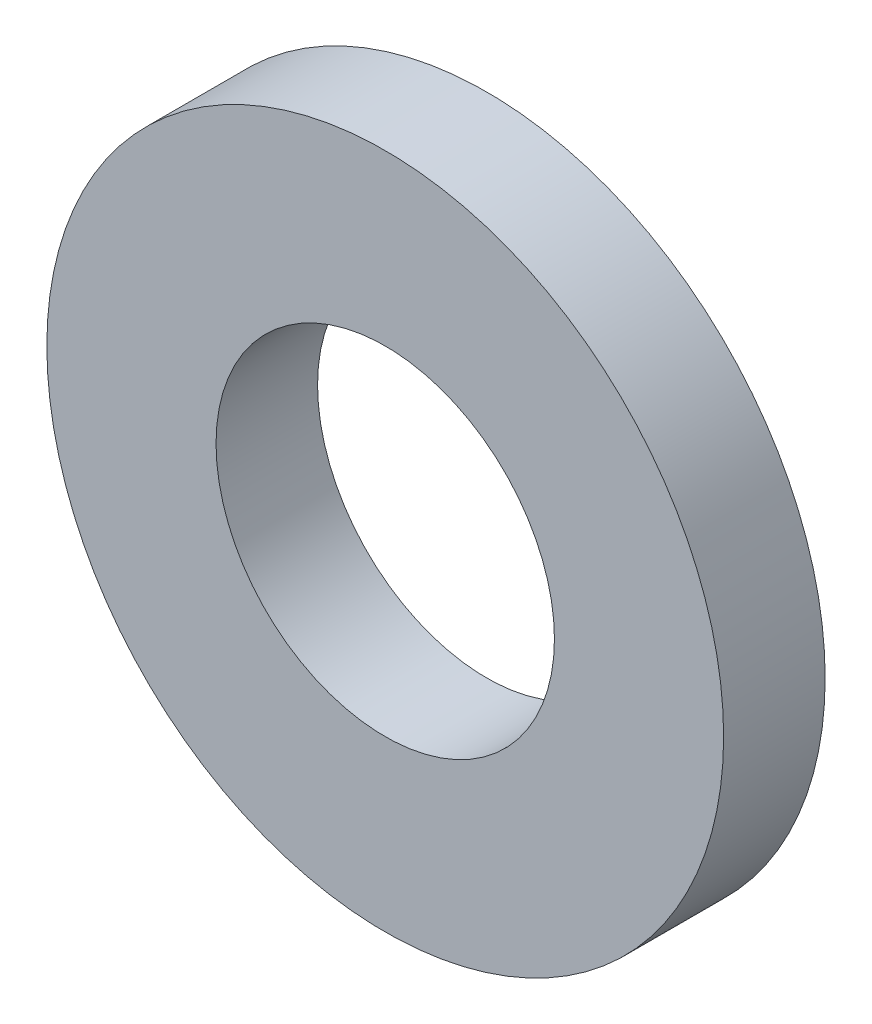
from build123d import *

# Parameters (mm, degrees)
SKETCH1_R           = 5
SKETCH1_R_2         = 2.5
BOSS_EXTRUDE1_DEPTH = 1.5


with BuildPart() as part:
    # Sketch1 → Boss-Extrude1 (new body)
    with BuildSketch(Plane.XY):
        Circle(SKETCH1_R)
        Circle(SKETCH1_R_2, mode=Mode.SUBTRACT)
    extrude(amount=BOSS_EXTRUDE1_DEPTH)


solid = part.part
